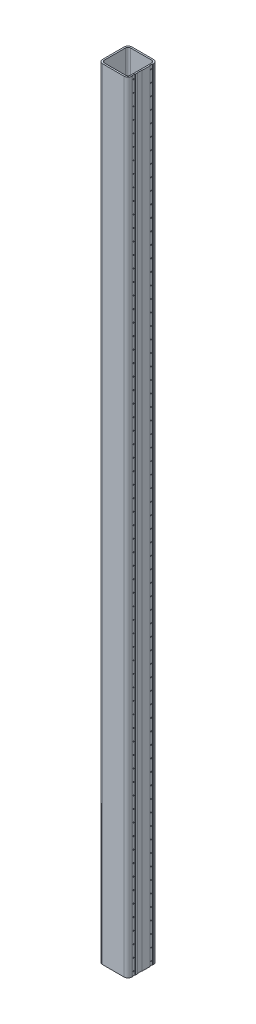
SolidWorks part; units mm, degrees
ref_plane "Front Plane" through (0, 0, 0) normal (0, 0, 1) x (1, 0, 0)
ref_plane "Top Plane" through (0, 0, 0) normal (0, 1, 0) x (1, 0, 0)
ref_plane "Right Plane" through (0, 0, 0) normal (1, 0, 0) x (0, 0, -1)
sketch "Sketch1" plane through (0, 0, 0) normal (0, 1, 0) x (1, 0, 0)
  line L0 (-67, -55) -> (-67, 55)
  line L1 (-55, -75) -> (55, -75)
  line L2 (-75, -55) -> (-75, 55)
  line L3 (-55, 75) -> (55, 75)
  line L4 (75, -55) -> (75, 55)
  line L5 (-75, -75) -> (75, 75) construction
  line L6 (-75, 75) -> (75, -75) construction
  line L7 (-55, 67) -> (55, 67)
  line L8 (67, -55) -> (67, 55)
  line L9 (-55, -67) -> (55, -67)
  arc A0 (55, -75) -> (75, -55) centre (55, -55) ccw
  arc A1 (55, 75) -> (75, 55) centre (55, 55) cw
  arc A2 (-75, 55) -> (-55, 75) centre (-55, 55) cw
  arc A3 (-55, -75) -> (-75, -55) centre (-55, -55) cw
  arc A4 (-67, 55) -> (-55, 67) centre (-55, 55) cw
  arc A5 (55, 67) -> (67, 55) centre (55, 55) cw
  arc A6 (55, -67) -> (67, -55) centre (55, -55) ccw
  arc A7 (-55, -67) -> (-67, -55) centre (-55, -55) cw
  point P0 (0, 0)
  dimension "D3" = 20
  dimension "D1" = 150
  dimension "D2" = 150
  dimension "D4" = 8
extrude "Boss-Extrude1" add sketch "Sketch1" along normal mid plane 4000
sketch "Sketch2" plane through (0, -2000, 0) normal (0, -1, 0) x (1, 0, 0)
  line L0 (75, 55) -> (75, -55) construction
  line L1 (75, 52.7) -> (73, 52.7)
  line L2 (75, 52.7) -> (75, 37.7)
  line L3 (75, 37.7) -> (73, 37.7)
  line L4 (73, 52.7) -> (73, 37.7)
  line L5 (0, 0) -> (75, 0) construction
  line L6 (75, -37.7) -> (73, -37.7)
  line L7 (75, -37.7) -> (75, -52.7)
  line L8 (75, -52.7) -> (73, -52.7)
  line L9 (73, -37.7) -> (73, -52.7)
  line L11 (75, 27.2) -> (73.5, 27.2)
  line L12 (75, 27.2) -> (75, 2.2)
  line L13 (75, 2.2) -> (73.5, 2.2)
  line L14 (73.5, 27.2) -> (73.5, 2.2)
  dimension "D1" = 2
  dimension "D2" = 15
  dimension "D3" = 15
  dimension "D4" = 2
  dimension "D5" = 37.7
  dimension "D6" = 37.7
  dimension "D7" = 1.5
  dimension "D8" = 25
  dimension "D9" = 10.5
extrude "Cut-Extrude1" cut sketch "Sketch2" against normal blind 4000
sketch "Sketch4" plane through (73, 0, 0) normal (1, 0, 0) x (0, 0, -1)
  line L0 (-52.7, -2000) -> (-37.7, -2000) construction
  circle A0 centre (-45.2, -1980) radius 2.6
  dimension "D1" = 5.2
  dimension "D2" = 20
  dimension "D3" = 45.2
extrude "Cut-Extrude2" cut sketch "Sketch4" against normal up to next
pattern_linear "LPattern2" count 2 spacing 90.4 along (0, 0, -1) count 67 spacing 60 along (0, 1, 0) of "Cut-Extrude2"
